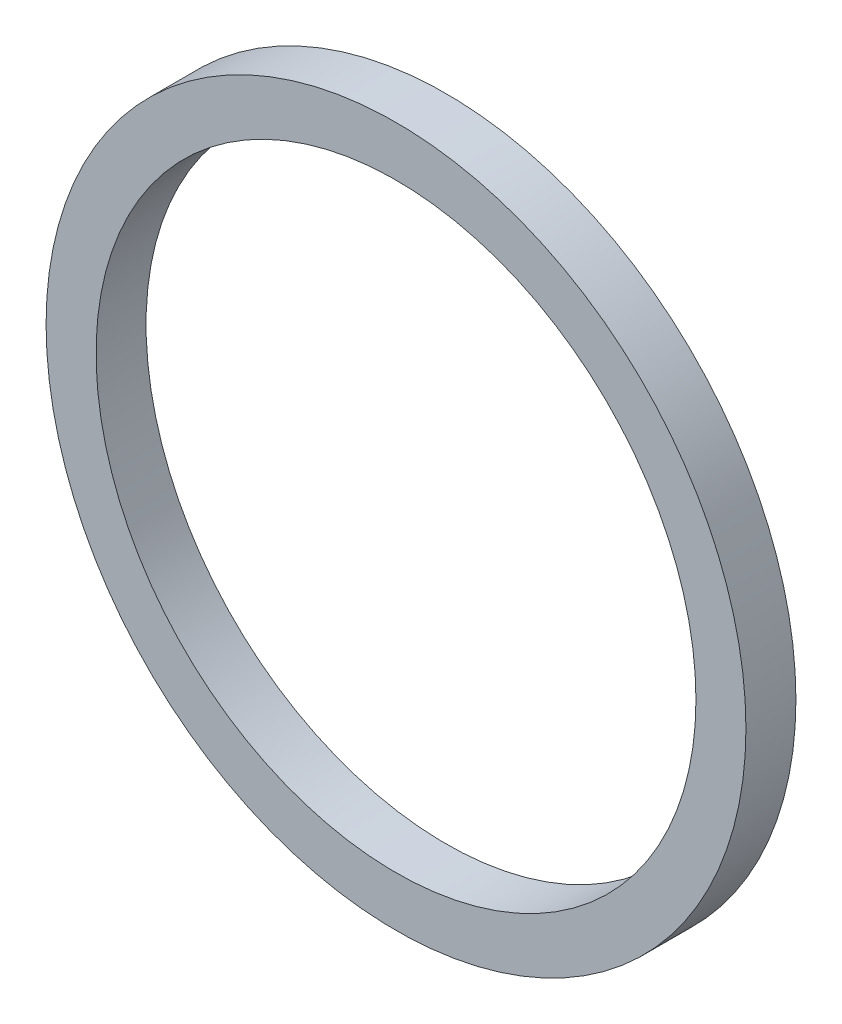
SolidWorks part; units mm, degrees
ref_plane "前视基准面" through (0, 0, 0) normal (0, 0, 1) x (1, 0, 0)
ref_plane "上视基准面" through (0, 0, 0) normal (0, 1, 0) x (1, 0, 0)
ref_plane "右视基准面" through (0, 0, 0) normal (1, 0, 0) x (0, 0, -1)
sketch "草图1" plane through (0, 0, 0) normal (0, 0, 1) x (1, 0, 0)
  circle A0 centre (0, 0) radius 17.5
  circle A1 centre (0, 0) radius 15
  point P4 (0, 0)
  dimension "D1" = 30
  dimension "D2" = 35
extrude "凸台-拉伸1" add sketch "草图1" along normal blind 2.5
